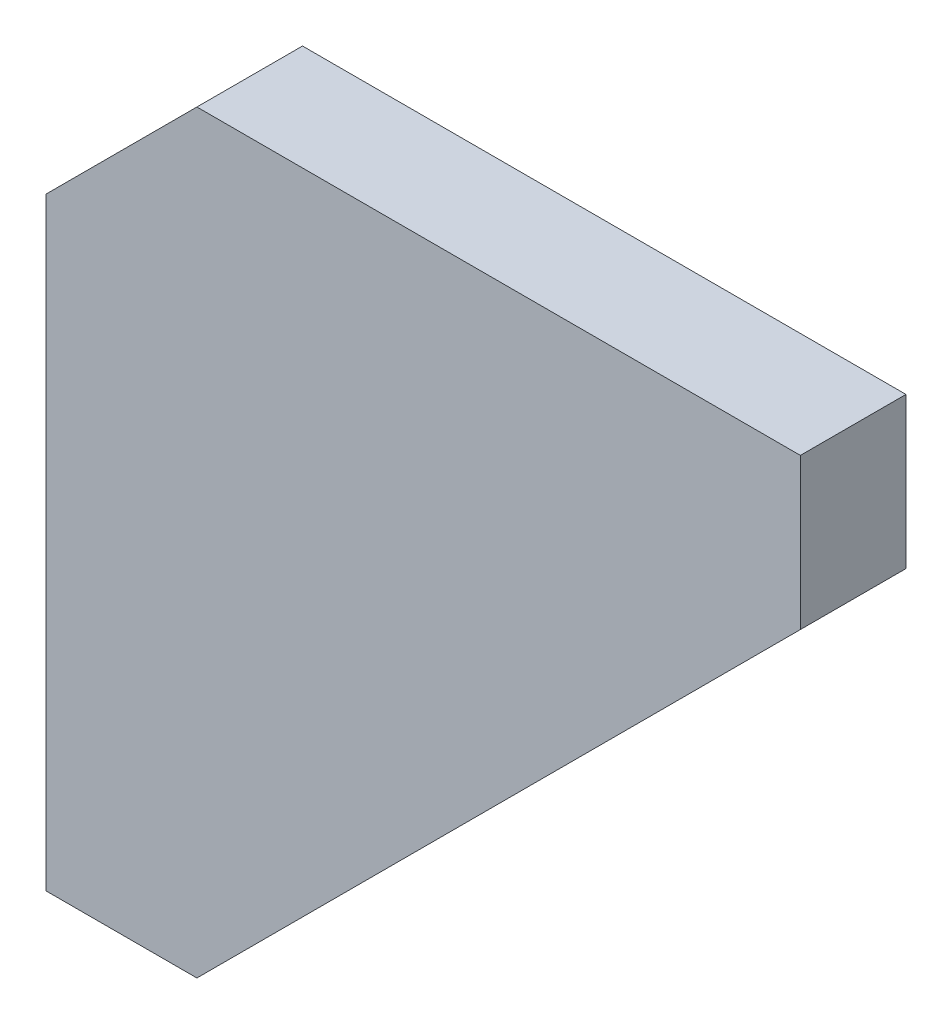
SolidWorks part; units mm, degrees
material "普通碳钢"
ref_plane "前视基准面" through (0, 0, 0) normal (0, 0, 1) x (1, 0, 0)
ref_plane "上视基准面" through (0, 0, 0) normal (0, 1, 0) x (1, 0, 0)
ref_plane "右视基准面" through (0, 0, 0) normal (1, 0, 0) x (0, 0, -1)
sketch "草图1" plane through (0, 0, 0) normal (0, 0, 1) x (1, 0, 0)
  line L0 (0, 0) -> (20, 0)
  line L1 (20, 0) -> (100, 80)
  line L2 (100, 80) -> (100, 100)
  line L3 (100, 100) -> (20, 100)
  line L4 (0, 80) -> (0, 0)
  line L5 (20, 100) -> (0, 80)
  point P6 (0, 100)
  dimension "D1" = 100
  dimension "D2" = 100
  dimension "D3" = 20
  dimension "D4" = 20
extrude "凸台-拉伸1" add sketch "草图1" along normal blind 14
